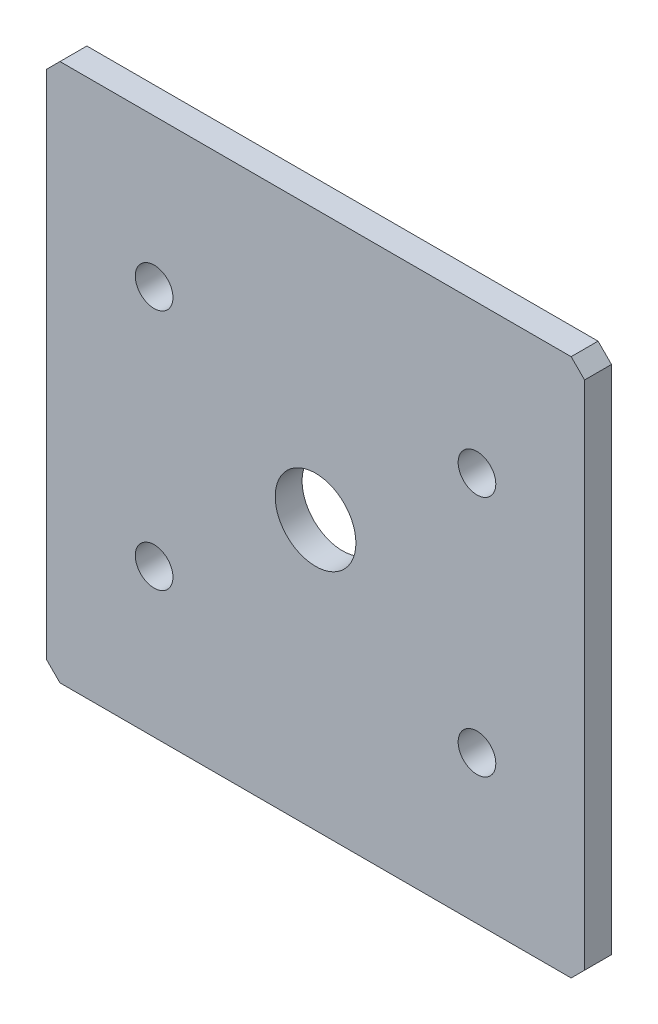
from build123d import *

# Parameters (mm, degrees)
SKETCH_1_W          = 200
SKETCH_1_H          = 200
EXTRUDE_1_DEPTH     = 10
SKETCH_2_R          = 7
SKETCH_2_R_2        = 15
CUT_EXTRUDE_1_DEPTH = 284.019433962
CHAMFER_1_SIZE      = 5


with BuildPart() as part:
    # 草图1 → 凸台-拉伸1 (new body)
    with BuildSketch(Plane.XY):
        with Locations((100, -100)):
            Rectangle(SKETCH_1_W, SKETCH_1_H)
    extrude(amount=EXTRUDE_1_DEPTH)

    # 草图2 → 切除-拉伸1 (cut, through all)
    with BuildSketch(Plane.XY.offset(10)):
        with Locations((40, -55)):
            Circle(SKETCH_2_R)
        with Locations((40, -145)):
            Circle(SKETCH_2_R)
        with Locations((160, -145)):
            Circle(SKETCH_2_R)
        with Locations((160, -55)):
            Circle(SKETCH_2_R)
        with Locations((100, -100)):
            Circle(SKETCH_2_R_2)
    extrude(amount=-CUT_EXTRUDE_1_DEPTH, mode=Mode.SUBTRACT)

    # 倒角1
    chamfer_1_edges = [part.edges().sort_by_distance(p)[0] for p in [
        (0, 0, 5),
        (200, 0, 5),
        (200, -200, 5),
        (0, -200, 5),
    ]]
    chamfer(chamfer_1_edges, length=CHAMFER_1_SIZE)


solid = part.part
